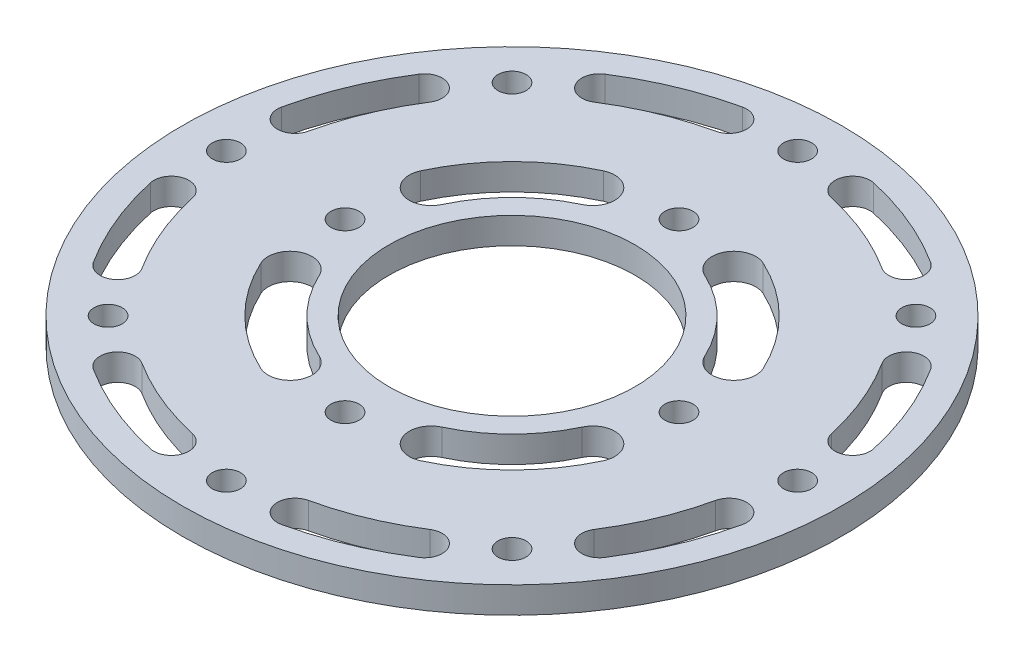
SolidWorks part; units mm, degrees
material "哈碳纤"
ref_plane "前视基准面" through (0, 0, 0) normal (0, 0, 1) x (1, 0, 0)
ref_plane "上视基准面" through (0, 0, 0) normal (0, 1, 0) x (1, 0, 0)
ref_plane "右视基准面" through (0, 0, 0) normal (1, 0, 0) x (0, 0, -1)
other "Configuration Table"
sketch "草图1" plane through (0, 0, 0) normal (0, 1, 0) x (1, 0, 0)
  circle A0 centre (0, 0) radius 32.5 construction
  circle A1 centre (0, 0) radius 37.5
  circle A2 centre (0, 0) radius 19 construction
  circle A3 centre (0, 19) radius 1.6
  circle A4 centre (19, 0) radius 1.6
  circle A5 centre (0, -19) radius 1.6
  circle A6 centre (-19, 0) radius 1.6
  circle A7 centre (0, 32.5) radius 1.6
  circle A8 centre (22.981, 22.981) radius 1.6
  circle A9 centre (32.5, 0) radius 1.6
  circle A10 centre (22.981, -22.981) radius 1.6
  circle A11 centre (0, -32.5) radius 1.6
  circle A12 centre (-22.981, -22.981) radius 1.6
  circle A13 centre (-32.5, 0) radius 1.6
  circle A14 centre (-22.981, 22.981) radius 1.6
  circle A15 centre (0, 0) radius 14
  point P16 (0, 0)
  dimension "D1" = 65
  dimension "D2" = 75
  dimension "D3" = 38
  dimension "D4" = 3.2
  dimension "D6" = 3.2
  dimension "D8" = 28
  dimension "D5" = 4
  dimension "D7" = 8
extrude "凸台-拉伸1" add sketch "草图1" along normal blind 3
sketch "草图2" plane through (0, 3, 0) normal (0, 1, 0) x (1, 0, 0)
  line L0 (-17.4622, 27.4102) -> (0, 0) construction
  line L1 (0, 0) -> (-7.0343, 31.7296) construction
  line L2 (-17.2198, 8.0297) -> (0, 0) construction
  line L3 (0, 0) -> (-8.0297, 17.2198) construction
  line L4 (-13.435, 13.435) -> (0, 0) construction
  line L5 (0, 0) -> (-12.4372, 30.0261) construction
  line L6 (0, -1000) -> (0, 49000) construction
  circle A0 centre (0, 0) radius 32.5 construction
  circle A1 centre (0, 0) radius 19 construction
  arc A2 (-17.4622, 27.4102) -> (-7.0343, 31.7296) centre (0, 0) cw construction
  arc A3 (-7.4672, 33.6822) -> (-18.5368, 29.097) centre (0, 0) ccw
  arc A4 (-6.6014, 29.777) -> (-16.3876, 25.7234) centre (0, 0) ccw
  arc A5 (-6.6014, 29.777) -> (-7.4672, 33.6822) centre (-7.0343, 31.7296) ccw
  arc A6 (-18.5368, 29.097) -> (-16.3876, 25.7234) centre (-17.4622, 27.4102) ccw
  arc A7 (-17.2198, 8.0297) -> (-8.0297, 17.2198) centre (0, 0) cw construction
  arc A8 (-9.0863, 19.4856) -> (-19.4856, 9.0863) centre (0, 0) ccw
  arc A9 (-6.9732, 14.9541) -> (-14.9541, 6.9732) centre (0, 0) ccw
  arc A10 (-6.9732, 14.9541) -> (-9.0863, 19.4856) centre (-8.0297, 17.2198) ccw
  arc A11 (-19.4856, 9.0863) -> (-14.9541, 6.9732) centre (-17.2198, 8.0297) ccw
  arc A12 (7.0343, 31.7296) -> (17.4622, 27.4102) centre (0, 0) cw construction
  arc A13 (18.5368, 29.097) -> (7.4672, 33.6822) centre (0, 0) ccw
  arc A14 (16.3876, 25.7234) -> (6.6014, 29.777) centre (0, 0) ccw
  arc A15 (16.3876, 25.7234) -> (18.5368, 29.097) centre (17.4622, 27.4102) ccw
  arc A16 (7.4672, 33.6822) -> (6.6014, 29.777) centre (7.0343, 31.7296) ccw
  arc A17 (27.4102, 17.4622) -> (31.7296, 7.0343) centre (0, 0) cw construction
  arc A18 (33.6822, 7.4672) -> (29.097, 18.5368) centre (0, 0) ccw
  arc A19 (29.777, 6.6014) -> (25.7234, 16.3876) centre (0, 0) ccw
  arc A20 (29.777, 6.6014) -> (33.6822, 7.4672) centre (31.7296, 7.0343) ccw
  arc A21 (29.097, 18.5368) -> (25.7234, 16.3876) centre (27.4102, 17.4622) ccw
  arc A22 (31.7296, -7.0343) -> (27.4102, -17.4622) centre (0, 0) cw construction
  arc A23 (29.097, -18.5368) -> (33.6822, -7.4672) centre (0, 0) ccw
  arc A24 (25.7234, -16.3876) -> (29.777, -6.6014) centre (0, 0) ccw
  arc A25 (25.7234, -16.3876) -> (29.097, -18.5368) centre (27.4102, -17.4622) ccw
  arc A26 (33.6822, -7.4672) -> (29.777, -6.6014) centre (31.7296, -7.0343) ccw
  arc A27 (17.4622, -27.4102) -> (7.0343, -31.7296) centre (0, 0) cw construction
  arc A28 (7.4672, -33.6822) -> (18.5368, -29.097) centre (0, 0) ccw
  arc A29 (6.6014, -29.777) -> (16.3876, -25.7234) centre (0, 0) ccw
  arc A30 (6.6014, -29.777) -> (7.4672, -33.6822) centre (7.0343, -31.7296) ccw
  arc A31 (18.5368, -29.097) -> (16.3876, -25.7234) centre (17.4622, -27.4102) ccw
  arc A32 (-7.0343, -31.7296) -> (-17.4622, -27.4102) centre (0, 0) cw construction
  arc A33 (-18.5368, -29.097) -> (-7.4672, -33.6822) centre (0, 0) ccw
  arc A34 (-16.3876, -25.7234) -> (-6.6014, -29.777) centre (0, 0) ccw
  arc A35 (-16.3876, -25.7234) -> (-18.5368, -29.097) centre (-17.4622, -27.4102) ccw
  arc A36 (-7.4672, -33.6822) -> (-6.6014, -29.777) centre (-7.0343, -31.7296) ccw
  arc A37 (-27.4102, -17.4622) -> (-31.7296, -7.0343) centre (0, 0) cw construction
  arc A38 (-33.6822, -7.4672) -> (-29.097, -18.5368) centre (0, 0) ccw
  arc A39 (-29.777, -6.6014) -> (-25.7234, -16.3876) centre (0, 0) ccw
  arc A40 (-29.777, -6.6014) -> (-33.6822, -7.4672) centre (-31.7296, -7.0343) ccw
  arc A41 (-29.097, -18.5368) -> (-25.7234, -16.3876) centre (-27.4102, -17.4622) ccw
  arc A42 (-31.7296, 7.0343) -> (-27.4102, 17.4622) centre (0, 0) cw construction
  arc A43 (-29.097, 18.5368) -> (-33.6822, 7.4672) centre (0, 0) ccw
  arc A44 (-25.7234, 16.3876) -> (-29.777, 6.6014) centre (0, 0) ccw
  arc A45 (-25.7234, 16.3876) -> (-29.097, 18.5368) centre (-27.4102, 17.4622) ccw
  arc A46 (-33.6822, 7.4672) -> (-29.777, 6.6014) centre (-31.7296, 7.0343) ccw
  arc A47 (8.0297, 17.2198) -> (17.2198, 8.0297) centre (0, 0) cw construction
  arc A48 (19.4856, 9.0863) -> (9.0863, 19.4856) centre (0, 0) ccw
  arc A49 (14.9541, 6.9732) -> (6.9732, 14.9541) centre (0, 0) ccw
  arc A50 (14.9541, 6.9732) -> (19.4856, 9.0863) centre (17.2198, 8.0297) ccw
  arc A51 (9.0863, 19.4856) -> (6.9732, 14.9541) centre (8.0297, 17.2198) ccw
  arc A52 (17.2198, -8.0297) -> (8.0297, -17.2198) centre (0, 0) cw construction
  arc A53 (9.0863, -19.4856) -> (19.4856, -9.0863) centre (0, 0) ccw
  arc A54 (6.9732, -14.9541) -> (14.9541, -6.9732) centre (0, 0) ccw
  arc A55 (6.9732, -14.9541) -> (9.0863, -19.4856) centre (8.0297, -17.2198) ccw
  arc A56 (19.4856, -9.0863) -> (14.9541, -6.9732) centre (17.2198, -8.0297) ccw
  arc A57 (-8.0297, -17.2198) -> (-17.2198, -8.0297) centre (0, 0) cw construction
  arc A58 (-19.4856, -9.0863) -> (-9.0863, -19.4856) centre (0, 0) ccw
  arc A59 (-14.9541, -6.9732) -> (-6.9732, -14.9541) centre (0, 0) ccw
  arc A60 (-14.9541, -6.9732) -> (-19.4856, -9.0863) centre (-17.2198, -8.0297) ccw
  arc A61 (-9.0863, -19.4856) -> (-6.9732, -14.9541) centre (-8.0297, -17.2198) ccw
  point P6 (-12.4372, 30.0261)
  point P14 (-13.435, 13.435)
  point P32 (12.4372, 30.0261)
  point P39 (30.0261, 12.4372)
  point P46 (30.0261, -12.4372)
  point P53 (12.4372, -30.0261)
  point P60 (-12.4372, -30.0261)
  point P67 (-30.0261, -12.4372)
  point P74 (-30.0261, 12.4372)
  point P79 (0, 0)
  point P83 (13.435, 13.435)
  point P90 (13.435, -13.435)
  point P97 (-13.435, -13.435)
  point P102 (0, 0)
  dimension "D1" = 65
  dimension "D2" = 38
  dimension "D3" = 20
  dimension "D7" = 4
  dimension "D8" = 5
  dimension "D4" = 22.5
  dimension "D5" = 45
  dimension "D6" = 40
  dimension "D9" = 8
  dimension "D10" = 4
extrude "切除-拉伸1" cut sketch "草图2" against normal through all both and the other way through all
